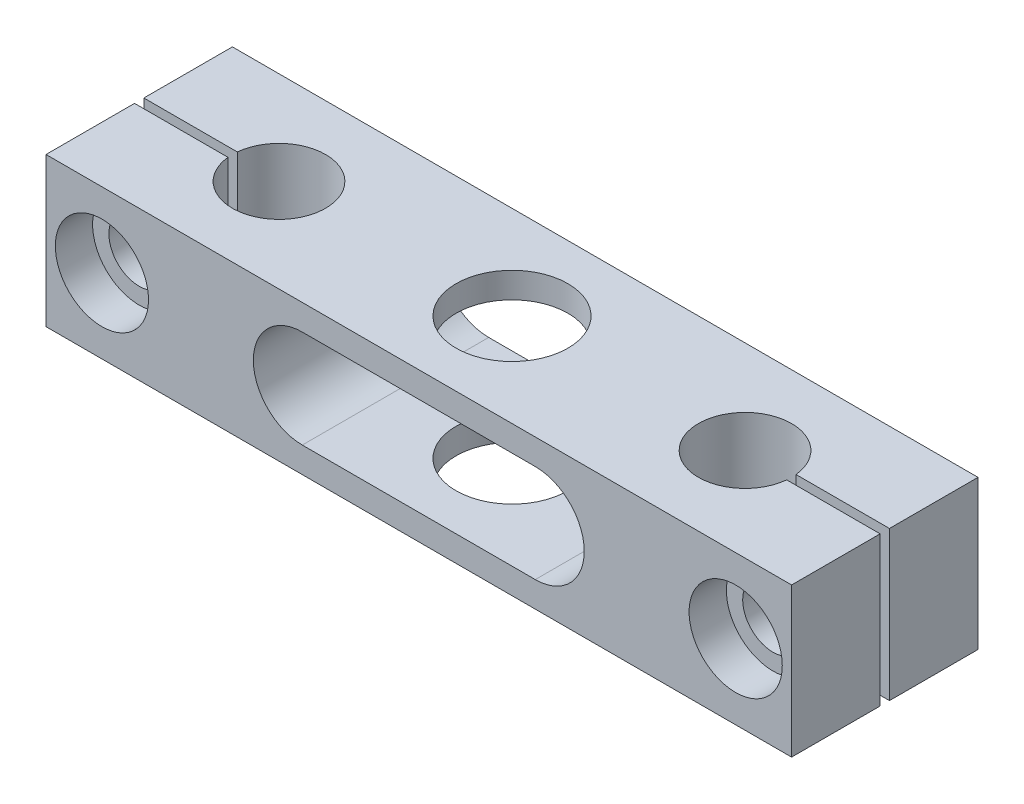
SolidWorks part; units mm, degrees
ref_plane "Front Plane" through (0, 0, 0) normal (0, 0, 1) x (1, 0, 0)
ref_plane "Top Plane" through (0, 0, 0) normal (0, 1, 0) x (1, 0, 0)
ref_plane "Right Plane" through (0, 0, 0) normal (1, 0, 0) x (0, 0, -1)
sketch "Sketch1" plane through (0, 0, 0) normal (0, 0, 1) x (1, 0, 0)
  line L0 (-3.1623, 11.7106) -> (21.8377, 11.7106)
  line L1 (-30.6623, -1.5394) -> (49.3377, -1.5394)
  line L2 (-30.6623, -1.5394) -> (-30.6623, 14.4606)
  line L3 (-30.6623, 14.4606) -> (49.3377, 14.4606)
  line L4 (49.3377, -1.5394) -> (49.3377, 14.4606)
  line L5 (-3.1623, 1.2106) -> (21.8377, 1.2106)
  arc A0 (21.8377, 1.2106) -> (21.8377, 11.7106) centre (21.8377, 6.4606) ccw
  arc A1 (-3.1623, 11.7106) -> (-3.1623, 1.2106) centre (-3.1623, 6.4606) ccw
  dimension "D3" = 10.5
  dimension "D4" = 8
  dimension "D5" = 27.5
  dimension "D6" = 8
  dimension "D7" = 25
  dimension "D1" = 80
  dimension "D2" = 16
  dimension "D9" = 27.5
extrude "Boss-Extrude1" add sketch "Sketch1" along normal blind 20
sketch "Sketch2" plane through (0, -1.5394, 0) normal (0, -1, 0) x (1, 0, 0)
  line L0 (-30.6623, 20) -> (-30.6623, 0) construction
  line L1 (-30.6623, 20) -> (49.3377, 20) construction
  line L3 (49.3377, 20) -> (49.3377, 0) construction
  circle A0 centre (34.3377, 10) radius 5
  circle A1 centre (-15.6623, 10) radius 5
  dimension "D1" = 10
  dimension "D2" = 10
  dimension "D3" = 15
  dimension "D4" = 10
  dimension "D5" = 10
  dimension "D6" = 15
extrude "Cut-Extrude1" cut sketch "Sketch2" against normal blind 20
sketch "Sketch4" plane through (0, 11.7106, 0) normal (0, -1, 0) x (1, 0, 0)
  line L0 (49.3377, 20) -> (49.3377, 0) construction
  line L1 (-30.6623, 0) -> (49.3377, 0) construction
  line L2 (-30.6623, 20) -> (49.3377, 20) construction
  circle A0 centre (9.3377, 10) radius 6
  dimension "D1" = 12
  dimension "D2" = 40
  dimension "D3" = 10
  dimension "D4" = 10
extrude "Cut-Extrude2" cut sketch "Sketch4" against normal mid plane 33
sketch "Sketch5" plane through (0, -1.5394, 0) normal (0, -1, 0) x (1, 0, 0)
  line L0 (34.3377, 10) -> (63.4438, 10) construction
  line L1 (-15.6623, 10) -> (-52.6988, 10) construction
  line L2 (34.3377, 9.5) -> (63.4438, 9.5)
  line L3 (34.3377, 10.5) -> (63.4438, 10.5)
  line L4 (-15.6623, 9.5) -> (-52.6988, 9.5)
  line L5 (-15.6623, 10.5) -> (-52.6988, 10.5)
  line L6 (-52.6988, 10.5) -> (-52.6988, 9.5)
  line L7 (-15.6623, 10.5) -> (-15.6623, 9.5)
  line L8 (63.4438, 10.5) -> (63.4438, 9.5)
  line L9 (34.3377, 10.5) -> (34.3377, 9.5)
  dimension "D1" = 0.5
  dimension "D2" = 0.5
  dimension "D3" = 0.5
  dimension "D4" = 0.5
extrude "Cut-Extrude3" cut sketch "Sketch5" against normal blind 30
hole_wizard "M6 Tapped Hole1" positions "Sketch7" profile "Sketch6" tap size "M6" standard "Gb"
sketch "Sketch7" plane through (0, 0, 9.5) normal (0, 0, 1) x (1, 0, 0)
  line L0 (49.3377, 14.4606) -> (-30.6623, 14.4606) construction
  line L1 (49.3377, -1.5394) -> (49.3377, 14.4606) construction
  line L2 (-30.6623, 14.4606) -> (-30.6623, -1.5394) construction
  point P0 (43.3377, 6.4606)
  point P2 (-24.6623, 6.4606)
  dimension "D1" = 8
  dimension "D2" = 8
  dimension "D3" = 6
  dimension "D4" = 6
sketch "Sketch6" plane through (43.3377, 6.4606, 9.5) normal (1, 0, 0) x (0, -1, 0)
  line L0 (0, 0) -> (0, 18.5022)
  line L1 (0, 18.5022) -> (2.5, 17)
  line L2 (2.5, 17) -> (2.5, 0)
  line L5 (2.5, 0) -> (0, 0)
  line L10 (0, 18.5022) -> (-2.5, 17) construction
  line L11 (0, -6.35) -> (0, 107.95) construction
  dimension "螺纹孔钻头直径" = 5
  dimension "螺纹孔钻头深度" = 17
  dimension "导头角度" = 118
cosmetic thread "CosmeticThread 1" parameters "D1"=9.5, "D2"=6
cosmetic thread "CosmeticThread 2" parameters "D1"=9.5, "D2"=6
sketch "Sketch8" plane through (0, 0, 10.5) normal (0, 0, -1) x (-1, 0, 0)
  circle A0 centre (24.6623, 6.4606) radius 3.25
  circle A1 centre (-43.3377, 6.4606) radius 3.25
  dimension "D1" = 6.5
  dimension "D2" = 6.5
extrude "Cut-Extrude4" cut sketch "Sketch8" against normal blind 30
sketch "Sketch9" plane through (0, 0, 20) normal (0, 0, 1) x (1, 0, 0)
  circle A0 centre (43.3377, 6.4606) radius 5
  circle A1 centre (-24.6623, 6.4606) radius 5
  dimension "D1" = 10
  dimension "D2" = 10
extrude "Cut-Extrude5" cut sketch "Sketch9" against normal blind 4
